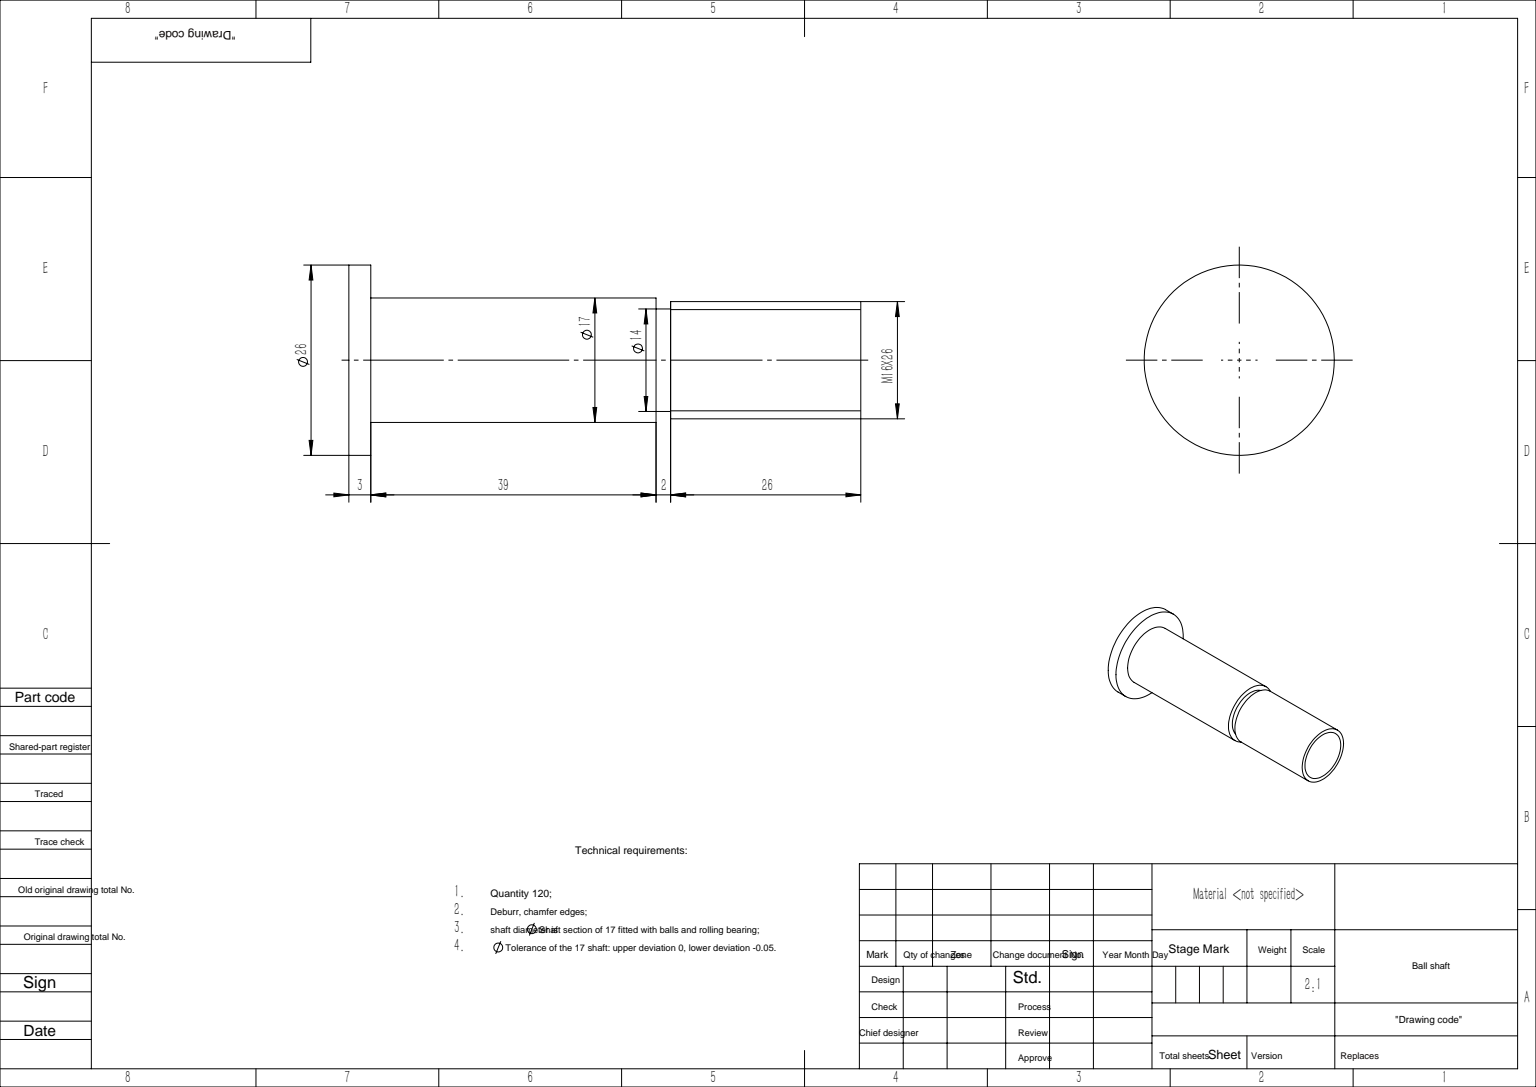
SolidWorks part; units mm, degrees
ref_plane "前视基准面" through (0, 0, 0) normal (0, 0, 1) x (1, 0, 0)
ref_plane "上视基准面" through (0, 0, 0) normal (0, 1, 0) x (1, 0, 0)
ref_plane "右视基准面" through (0, 0, 0) normal (1, 0, 0) x (0, 0, -1)
sketch "草图1" plane through (0, 0, 0) normal (0, 0, 1) x (1, 0, 0)
  line L0 (0, 0) -> (100, 0) construction
  line L1 (0, 0) -> (0, 13)
  line L2 (0, 13) -> (3, 13)
  line L3 (3, 13) -> (3, 8.5)
  line L4 (3, 8.5) -> (70, 8.5)
  line L5 (70, 8.5) -> (70, 0)
  line L6 (70, 0) -> (0, 0)
  dimension "D1" = 8.5
  dimension "D2" = 13
  dimension "D3" = 3
  dimension "D4" = 67
  dimension "D5" = 100
revolve "旋转1" add sketch "草图1" angle 360 about L0
sketch "草图2" plane through (70, 0, 0) normal (1, 0, 0) x (0, 0, -1)
  circle A0 centre (0, 0) radius 8
  circle A1 centre (0, 0) radius 8.5 construction
  circle A2 centre (0, 0) radius 8.5
  dimension "D1" = 16
extrude "切除-拉伸1" cut sketch "草图2" against normal blind 28
cosmetic thread "装饰螺纹线3" parameters "D1"=26, "D2"=13.835
sketch "草图3" plane through (42, 0, 0) normal (1, 0, 0) x (0, 0, -1)
  circle A1 centre (0, 0) radius 8 construction
  circle A2 centre (0, 0) radius 8
  circle A3 centre (0, 0) radius 7
  dimension "D1" = 1
extrude "切除-拉伸2" cut sketch "草图3" along normal blind 2
